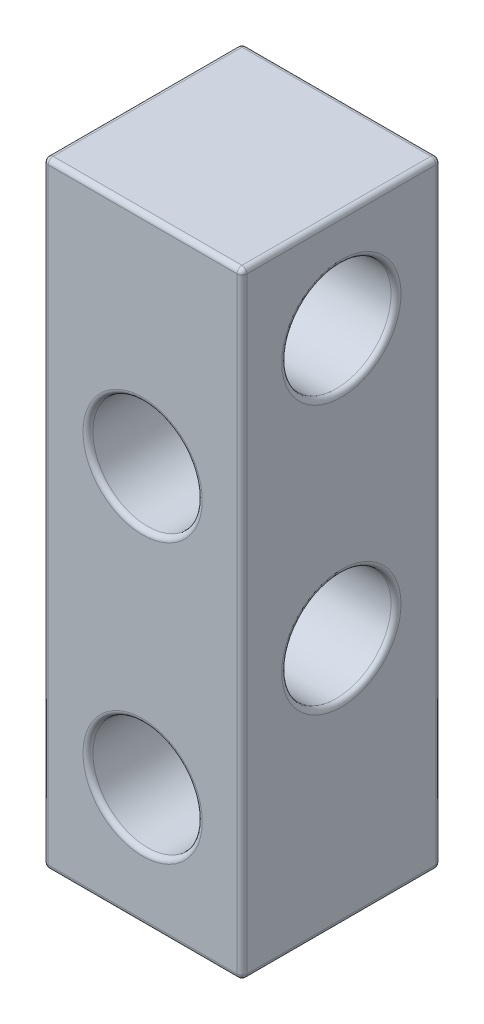
from build123d import *

# Parameters (mm, degrees)
SKETCH1_W           = 20
SKETCH1_H           = 62
SKETCH1_R           = 5.5
BOSS_EXTRUDE1_DEPTH = 10
SKETCH2_R           = 5.5
CUT_EXTRUDE1_DEPTH  = 20
FILLET1_R           = 0.5


with BuildPart() as part:
    # Sketch1 → Boss-Extrude1 (new, symmetric)
    with BuildSketch(Plane.XY):
        Rectangle(SKETCH1_W, SKETCH1_H)
        with Locations((0, -19)):
            Circle(SKETCH1_R, mode=Mode.SUBTRACT)
        with Locations((0, 9)):
            Circle(SKETCH1_R, mode=Mode.SUBTRACT)
    extrude(amount=BOSS_EXTRUDE1_DEPTH, both=True)

    # Sketch2 → Cut-Extrude1 (cut)
    with BuildSketch(Plane(origin=(10, 0, 0), x_dir=(0, 0, -1), z_dir=(1, 0, 0))):
        with Locations((0, 21)):
            Circle(SKETCH2_R)
        with Locations((0, -6)):
            Circle(SKETCH2_R)
    extrude(amount=-CUT_EXTRUDE1_DEPTH, mode=Mode.SUBTRACT)

    # Fillet1
    fillet1_edges = [part.edges().sort_by_distance(p)[0] for p in [
        (10, 0, 10),
        (-5.5, -19, -10),
        (-5.5, -19, 10),
        (0, 31, 10),
        (-5.5, 9, -10),
        (-5.5, 9, 10),
        (-10, 21, 5.5),
        (10, 21, 5.5),
        (-10, -6, 5.5),
        (10, -6, 5.5),
        (-10, 0, 10),
        (0, 31, -10),
        (10, 0, -10),
        (0, -31, -10),
        (-10, 0, -10),
        (0, -31, 10),
        (-10, 31, 0),
        (10, 31, 0),
        (10, -31, 0),
        (-10, -31, 0),
    ]]
    fillet(fillet1_edges, radius=FILLET1_R)


solid = part.part
